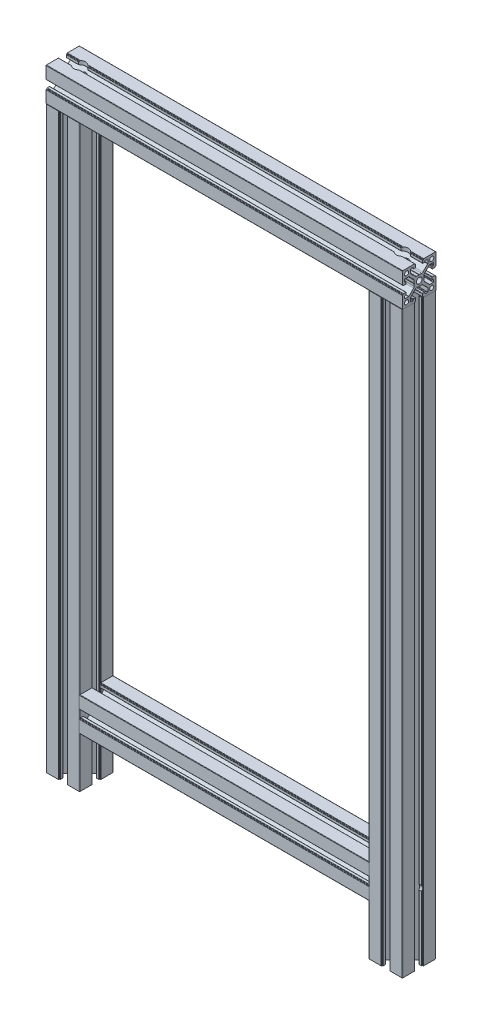
SolidWorks part; units mm, degrees
material "6061 合金"
ref_plane "前视基准面" through (0, 0, 0) normal (0, 0, 1) x (1, 0, 0)
ref_plane "上视基准面" through (0, 0, 0) normal (0, 1, 0) x (1, 0, 0)
ref_plane "右视基准面" through (0, 0, 0) normal (1, 0, 0) x (0, 0, -1)
sketch "草图1" plane through (0, 0, 0) normal (0, 0, 1) x (1, 0, 0)
  line L0 (192.5, 0) -> (-192.5, 0) construction
  line L1 (-192.5, 0) -> (-192.5, 710.5)
  line L2 (-212.5, 710.5) -> (212.5, 710.5)
  line L4 (0, 710.5) -> (0, 0) construction
  line L5 (-192.5, 80) -> (192.5, 80)
  line L8 (192.5, 0) -> (192.5, 710.5)
  dimension "D1" = 20
  dimension "D2" = 425
  dimension "D3" = 710.5
  dimension "D4" = 80
other "LE-8-4040HW"
ref_plane "基准面4" through (-212.5, 710.5, 0) normal (1, 0, 0) x (0, 1, 0)
sketch "草图14" plane through (-212.5, 710.5, 0) normal (1, 0, 0) x (0, 1, 0)
  line L0 (-6, -0.3) -> (-6, -3.0503)
  line L1 (-6.5858, -4.4645) -> (-12.2249, -10.1036)
  line L2 (-12.5784, -10.25) -> (-16.8, -10.25)
  line L3 (-17.3, -9.75) -> (-17.3, -7.6)
  line L4 (-16.8, -7.1) -> (-16, -7.1)
  line L5 (-15.5, -6.6) -> (-15.5, -4.6)
  line L6 (-16, -4.1) -> (-18.7, -4.1)
  line L7 (-19, -4.4) -> (-19, -4.8)
  line L8 (-19.3, -5.1) -> (-19.7, -5.1)
  line L9 (-20, -5.4) -> (-20, -19.5)
  line L10 (-19.5, -20) -> (-5.4, -20)
  line L11 (-5.1, -19.7) -> (-5.1, -19.3)
  line L12 (-4.8, -19) -> (-4.4, -19)
  line L13 (-4.1, -18.7) -> (-4.1, -16)
  line L14 (-4.6, -15.5) -> (-6.6, -15.5)
  line L15 (-7.1, -16) -> (-7.1, -16.8)
  line L16 (-7.6, -17.3) -> (-9.75, -17.3)
  line L17 (-10.25, -16.8) -> (-10.25, -12.5784)
  line L18 (-10.1036, -12.2249) -> (-4.4645, -6.5858)
  line L19 (-3.0503, -6) -> (-0.3, -6)
  line L20 (0.3, -6) -> (3.0503, -6)
  line L21 (4.4645, -6.5858) -> (10.1036, -12.2249)
  line L22 (10.25, -12.5784) -> (10.25, -16.8)
  line L23 (9.75, -17.3) -> (7.6, -17.3)
  line L24 (7.1, -16.8) -> (7.1, -16)
  line L25 (6.6, -15.5) -> (4.6, -15.5)
  line L26 (4.1, -16) -> (4.1, -18.7)
  line L27 (4.4, -19) -> (4.8, -19)
  line L28 (5.1, -19.3) -> (5.1, -19.7)
  line L29 (5.4, -20) -> (19.5, -20)
  line L30 (20, -19.5) -> (20, -5.4)
  line L31 (19.7, -5.1) -> (19.3, -5.1)
  line L32 (19, -4.8) -> (19, -4.4)
  line L33 (18.7, -4.1) -> (16, -4.1)
  line L34 (15.5, -4.6) -> (15.5, -6.6)
  line L35 (16, -7.1) -> (16.8, -7.1)
  line L36 (17.3, -7.6) -> (17.3, -9.75)
  line L37 (16.8, -10.25) -> (12.5784, -10.25)
  line L38 (12.2249, -10.1036) -> (6.5858, -4.4645)
  line L39 (6, -3.0503) -> (6, -0.3)
  line L40 (6, 0.3) -> (6, 3.0503)
  line L41 (6.5858, 4.4645) -> (12.2249, 10.1036)
  line L42 (12.5784, 10.25) -> (16.8, 10.25)
  line L43 (17.3, 9.75) -> (17.3, 7.6)
  line L44 (16.8, 7.1) -> (16, 7.1)
  line L45 (15.5, 6.6) -> (15.5, 4.6)
  line L46 (16, 4.1) -> (18.7, 4.1)
  line L47 (19, 4.4) -> (19, 4.8)
  line L48 (19.3, 5.1) -> (19.7, 5.1)
  line L49 (20, 5.4) -> (20, 19.5)
  line L50 (19.5, 20) -> (5.4, 20)
  line L51 (5.1, 19.7) -> (5.1, 19.3)
  line L52 (4.8, 19) -> (4.4, 19)
  line L53 (4.1, 18.7) -> (4.1, 16)
  line L54 (4.6, 15.5) -> (6.6, 15.5)
  line L55 (7.1, 16) -> (7.1, 16.8)
  line L56 (7.6, 17.3) -> (9.75, 17.3)
  line L57 (10.25, 16.8) -> (10.25, 12.5784)
  line L58 (10.1036, 12.2249) -> (4.4645, 6.5858)
  line L59 (3.0503, 6) -> (0.3, 6)
  line L60 (-0.3, 6) -> (-3.0503, 6)
  line L61 (-4.4645, 6.5858) -> (-10.1036, 12.2249)
  line L62 (-10.25, 12.5784) -> (-10.25, 16.8)
  line L63 (-9.75, 17.3) -> (-7.6, 17.3)
  line L64 (-7.1, 16.8) -> (-7.1, 16)
  line L65 (-6.6, 15.5) -> (-4.6, 15.5)
  line L66 (-4.1, 16) -> (-4.1, 18.7)
  line L67 (-4.4, 19) -> (-4.8, 19)
  line L68 (-5.1, 19.3) -> (-5.1, 19.7)
  line L69 (-5.4, 20) -> (-19.5, 20)
  line L70 (-20, 19.5) -> (-20, 5.4)
  line L71 (-19.7, 5.1) -> (-19.3, 5.1)
  line L72 (-19, 4.8) -> (-19, 4.4)
  line L73 (-18.7, 4.1) -> (-16, 4.1)
  line L74 (-15.5, 4.6) -> (-15.5, 6.6)
  line L75 (-16, 7.1) -> (-16.8, 7.1)
  line L76 (-17.3, 7.6) -> (-17.3, 9.75)
  line L77 (-16.8, 10.25) -> (-12.5784, 10.25)
  line L78 (-12.2249, 10.1036) -> (-6.5858, 4.4645)
  line L79 (-6, 3.0503) -> (-6, 0.3)
  circle A0 centre (-15, 15) radius 2.45
  circle A1 centre (0, 0) radius 3.4
  circle A2 centre (15, 15) radius 2.45
  circle A3 centre (15, -15) radius 2.45
  circle A4 centre (-15, -15) radius 2.45
  arc A5 (-6, -0.3) -> (-6, 0.3) centre (-6, 0) ccw
  arc A6 (-6.5858, -4.4645) -> (-6, -3.0503) centre (-8, -3.0503) ccw
  arc A7 (-12.5784, -10.25) -> (-12.2249, -10.1036) centre (-12.5784, -9.75) ccw
  arc A8 (-17.3, -9.75) -> (-16.8, -10.25) centre (-16.8, -9.75) ccw
  arc A9 (-16.8, -7.1) -> (-17.3, -7.6) centre (-16.8, -7.6) ccw
  arc A10 (-16, -7.1) -> (-15.5, -6.6) centre (-16, -6.6) ccw
  arc A11 (-15.5, -4.6) -> (-16, -4.1) centre (-16, -4.6) ccw
  arc A12 (-18.7, -4.1) -> (-19, -4.4) centre (-18.7, -4.4) ccw
  arc A13 (-19.3, -5.1) -> (-19, -4.8) centre (-19.3, -4.8) ccw
  arc A14 (-19.7, -5.1) -> (-20, -5.4) centre (-19.7, -5.4) ccw
  arc A15 (-20, -19.5) -> (-19.5, -20) centre (-19.5, -19.5) ccw
  arc A16 (-5.4, -20) -> (-5.1, -19.7) centre (-5.4, -19.7) ccw
  arc A17 (-4.8, -19) -> (-5.1, -19.3) centre (-4.8, -19.3) ccw
  arc A18 (-4.4, -19) -> (-4.1, -18.7) centre (-4.4, -18.7) ccw
  arc A19 (-4.1, -16) -> (-4.6, -15.5) centre (-4.6, -16) ccw
  arc A20 (-6.6, -15.5) -> (-7.1, -16) centre (-6.6, -16) ccw
  arc A21 (-7.6, -17.3) -> (-7.1, -16.8) centre (-7.6, -16.8) ccw
  arc A22 (-10.25, -16.8) -> (-9.75, -17.3) centre (-9.75, -16.8) ccw
  arc A23 (-10.1036, -12.2249) -> (-10.25, -12.5784) centre (-9.75, -12.5784) ccw
  arc A24 (-3.0503, -6) -> (-4.4645, -6.5858) centre (-3.0503, -8) ccw
  arc A25 (0.3, -6) -> (-0.3, -6) centre (0, -6) ccw
  arc A26 (4.4645, -6.5858) -> (3.0503, -6) centre (3.0503, -8) ccw
  arc A27 (10.25, -12.5784) -> (10.1036, -12.2249) centre (9.75, -12.5784) ccw
  arc A28 (9.75, -17.3) -> (10.25, -16.8) centre (9.75, -16.8) ccw
  arc A29 (7.1, -16.8) -> (7.6, -17.3) centre (7.6, -16.8) ccw
  arc A30 (7.1, -16) -> (6.6, -15.5) centre (6.6, -16) ccw
  arc A31 (4.6, -15.5) -> (4.1, -16) centre (4.6, -16) ccw
  arc A32 (4.1, -18.7) -> (4.4, -19) centre (4.4, -18.7) ccw
  arc A33 (5.1, -19.3) -> (4.8, -19) centre (4.8, -19.3) ccw
  arc A34 (5.1, -19.7) -> (5.4, -20) centre (5.4, -19.7) ccw
  arc A35 (19.5, -20) -> (20, -19.5) centre (19.5, -19.5) ccw
  arc A36 (20, -5.4) -> (19.7, -5.1) centre (19.7, -5.4) ccw
  arc A37 (19, -4.8) -> (19.3, -5.1) centre (19.3, -4.8) ccw
  arc A38 (19, -4.4) -> (18.7, -4.1) centre (18.7, -4.4) ccw
  arc A39 (16, -4.1) -> (15.5, -4.6) centre (16, -4.6) ccw
  arc A40 (15.5, -6.6) -> (16, -7.1) centre (16, -6.6) ccw
  arc A41 (17.3, -7.6) -> (16.8, -7.1) centre (16.8, -7.6) ccw
  arc A42 (16.8, -10.25) -> (17.3, -9.75) centre (16.8, -9.75) ccw
  arc A43 (12.2249, -10.1036) -> (12.5784, -10.25) centre (12.5784, -9.75) ccw
  arc A44 (6, -3.0503) -> (6.5858, -4.4645) centre (8, -3.0503) ccw
  arc A45 (6, 0.3) -> (6, -0.3) centre (6, 0) ccw
  arc A46 (6.5858, 4.4645) -> (6, 3.0503) centre (8, 3.0503) ccw
  arc A47 (12.5784, 10.25) -> (12.2249, 10.1036) centre (12.5784, 9.75) ccw
  arc A48 (17.3, 9.75) -> (16.8, 10.25) centre (16.8, 9.75) ccw
  arc A49 (16.8, 7.1) -> (17.3, 7.6) centre (16.8, 7.6) ccw
  arc A50 (16, 7.1) -> (15.5, 6.6) centre (16, 6.6) ccw
  arc A51 (15.5, 4.6) -> (16, 4.1) centre (16, 4.6) ccw
  arc A52 (18.7, 4.1) -> (19, 4.4) centre (18.7, 4.4) ccw
  arc A53 (19.3, 5.1) -> (19, 4.8) centre (19.3, 4.8) ccw
  arc A54 (19.7, 5.1) -> (20, 5.4) centre (19.7, 5.4) ccw
  arc A55 (20, 19.5) -> (19.5, 20) centre (19.5, 19.5) ccw
  arc A56 (5.4, 20) -> (5.1, 19.7) centre (5.4, 19.7) ccw
  arc A57 (4.8, 19) -> (5.1, 19.3) centre (4.8, 19.3) ccw
  arc A58 (4.4, 19) -> (4.1, 18.7) centre (4.4, 18.7) ccw
  arc A59 (4.1, 16) -> (4.6, 15.5) centre (4.6, 16) ccw
  arc A60 (6.6, 15.5) -> (7.1, 16) centre (6.6, 16) ccw
  arc A61 (7.6, 17.3) -> (7.1, 16.8) centre (7.6, 16.8) ccw
  arc A62 (10.25, 16.8) -> (9.75, 17.3) centre (9.75, 16.8) ccw
  arc A63 (10.1036, 12.2249) -> (10.25, 12.5784) centre (9.75, 12.5784) ccw
  arc A64 (3.0503, 6) -> (4.4645, 6.5858) centre (3.0503, 8) ccw
  arc A65 (-0.3, 6) -> (0.3, 6) centre (0, 6) ccw
  arc A66 (-4.4645, 6.5858) -> (-3.0503, 6) centre (-3.0503, 8) ccw
  arc A67 (-10.25, 12.5784) -> (-10.1036, 12.2249) centre (-9.75, 12.5784) ccw
  arc A68 (-9.75, 17.3) -> (-10.25, 16.8) centre (-9.75, 16.8) ccw
  arc A69 (-7.1, 16.8) -> (-7.6, 17.3) centre (-7.6, 16.8) ccw
  arc A70 (-7.1, 16) -> (-6.6, 15.5) centre (-6.6, 16) ccw
  arc A71 (-4.6, 15.5) -> (-4.1, 16) centre (-4.6, 16) ccw
  arc A72 (-4.1, 18.7) -> (-4.4, 19) centre (-4.4, 18.7) ccw
  arc A73 (-5.1, 19.3) -> (-4.8, 19) centre (-4.8, 19.3) ccw
  arc A74 (-5.1, 19.7) -> (-5.4, 20) centre (-5.4, 19.7) ccw
  arc A75 (-19.5, 20) -> (-20, 19.5) centre (-19.5, 19.5) ccw
  arc A76 (-20, 5.4) -> (-19.7, 5.1) centre (-19.7, 5.4) ccw
  arc A77 (-19, 4.8) -> (-19.3, 5.1) centre (-19.3, 4.8) ccw
  arc A78 (-19, 4.4) -> (-18.7, 4.1) centre (-18.7, 4.4) ccw
  arc A79 (-16, 4.1) -> (-15.5, 4.6) centre (-16, 4.6) ccw
  arc A80 (-15.5, 6.6) -> (-16, 7.1) centre (-16, 6.6) ccw
  arc A81 (-17.3, 7.6) -> (-16.8, 7.1) centre (-16.8, 7.6) ccw
  arc A82 (-16.8, 10.25) -> (-17.3, 9.75) centre (-16.8, 9.75) ccw
  arc A83 (-12.2249, 10.1036) -> (-12.5784, 10.25) centre (-12.5784, 9.75) ccw
  arc A84 (-6, 3.0503) -> (-6.5858, 4.4645) centre (-8, 3.0503) ccw
  point P250 (0, 0)
sketch "草图15" plane through (-212.5, 0, 0) normal (-1, 0, 0) x (0, 0, 1)
  circle A0 centre (0, 80) radius 4.4
extrude "切除-拉伸1" cut sketch "草图15" against normal blind 46 contours A0
sketch "草图16" plane through (212.5, 0, 0) normal (1, 0, 0) x (0, 0, -1)
  circle A0 centre (0, 80) radius 5.1
extrude "切除-拉伸3" cut sketch "草图16" against normal blind 40 contours A0
sketch "草图18" plane through (0, 730.5, 0) normal (0, 1, 0) x (1, 0, 0)
  line L0 (-212.5, 19.5) -> (-212.5, 5.4) construction
  circle A0 centre (192.5, 0) radius 7
  circle A1 centre (-192.5, 0) radius 7
  dimension "D5" = 14
  dimension "D6" = 14
  dimension "D1" = 20
  dimension "D2" = 20
  dimension "D3" = 20
  dimension "D4" = 20
extrude "切除-拉伸8" cut sketch "草图18" against normal blind 30
